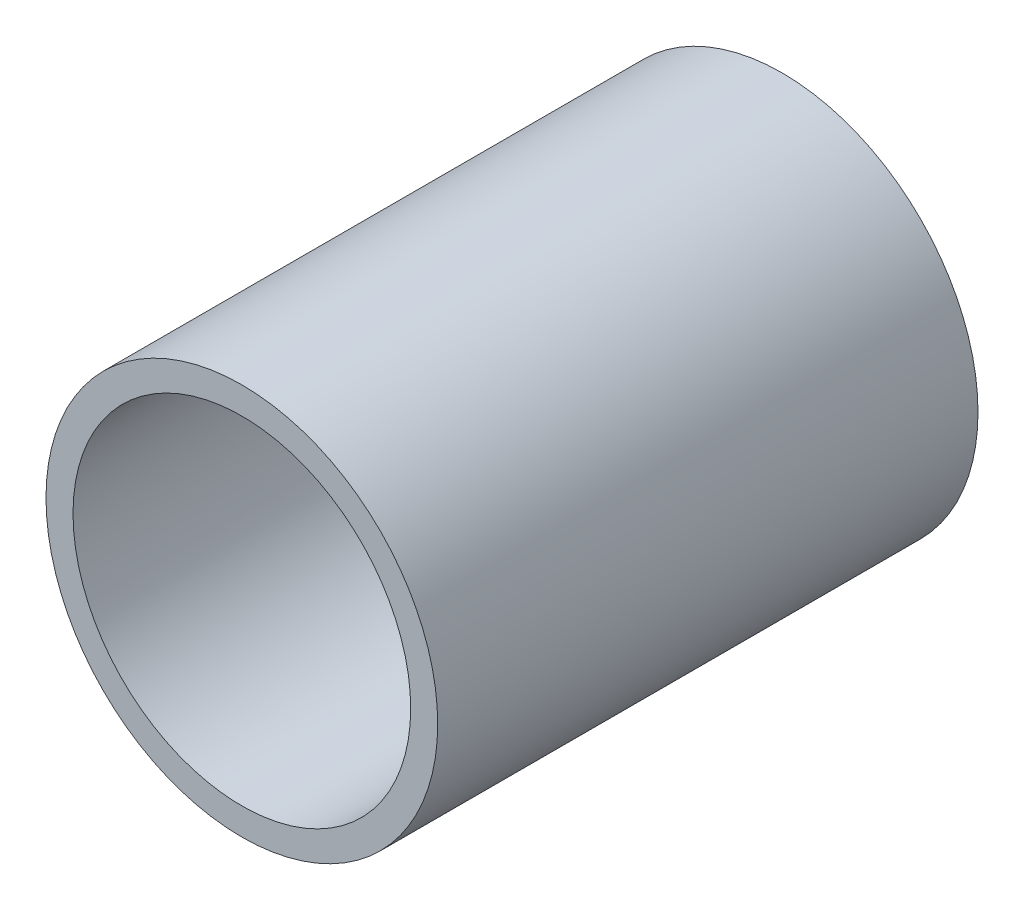
from build123d import *

# Parameters (mm, degrees)
SKETCH1_R           = 14.5
SKETCH1_R_2         = 12.5
BOSS_EXTRUDE1_DEPTH = 40


with BuildPart() as part:
    # Sketch1 → Boss-Extrude1 (new body)
    with BuildSketch(Plane.XY):
        Circle(SKETCH1_R)
        Circle(SKETCH1_R_2, mode=Mode.SUBTRACT)
    extrude(amount=BOSS_EXTRUDE1_DEPTH)


solid = part.part
